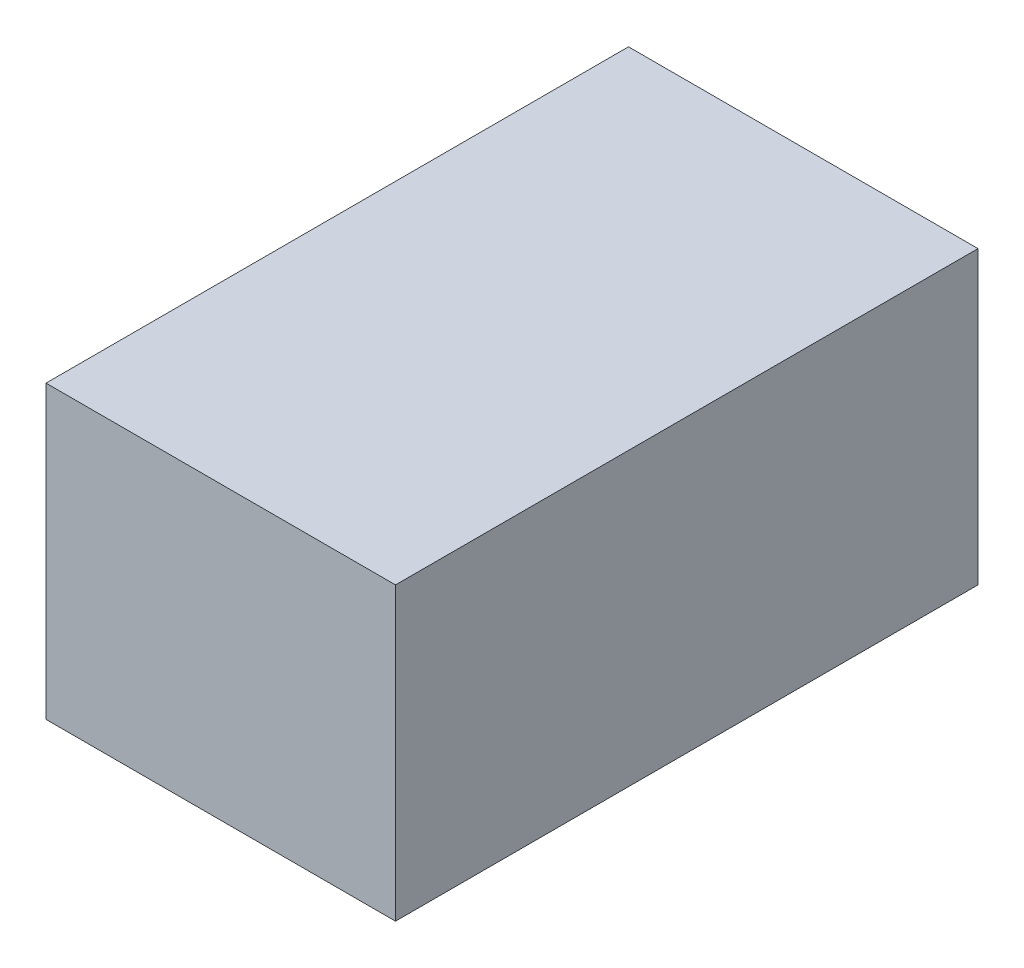
from build123d import *

# Parameters (mm, degrees)
SKETCH1_W           = 60
SKETCH1_H           = 100
BOSS_EXTRUDE1_DEPTH = 50


with BuildPart() as part:
    # Sketch1 → Boss-Extrude1 (new body)
    with BuildSketch(Plane(origin=(0, 0, 0), x_dir=(1, 0, 0), z_dir=(0, 1, 0))):
        Rectangle(SKETCH1_W, SKETCH1_H)
    extrude(amount=BOSS_EXTRUDE1_DEPTH)


solid = part.part
